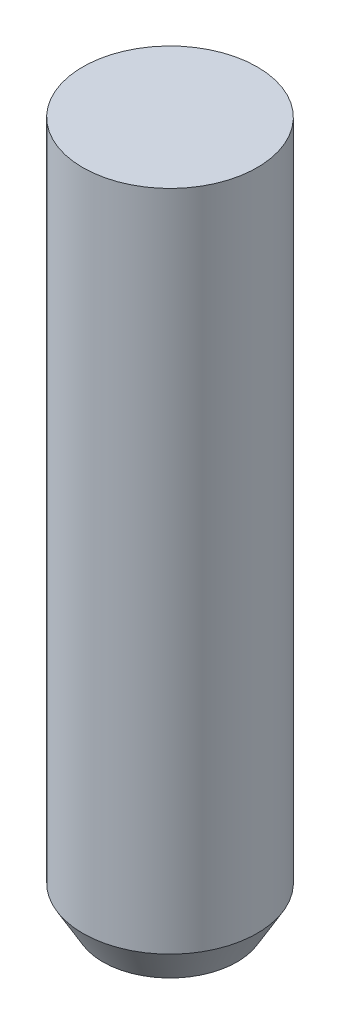
SolidWorks part; units mm, degrees
material "AISI 1045 钢，冷拔"
ref_plane "Front Plane" through (0, 0, 0) normal (0, 0, 1) x (1, 0, 0)
ref_plane "Top Plane" through (0, 0, 0) normal (0, 1, 0) x (1, 0, 0)
ref_plane "Right Plane" through (0, 0, 0) normal (1, 0, 0) x (0, 0, -1)
sketch "Sketch1" plane through (0, 0, 0) normal (0, 1, 0) x (1, 0, 0)
  circle A0 centre (0, 0) radius 5
extrude "Boss-Extrude1" add sketch "Sketch1" along normal blind 40
chamfer "Chamfer1" distance 1.1547 angle 60 1 edges at (0, 0, 5)
